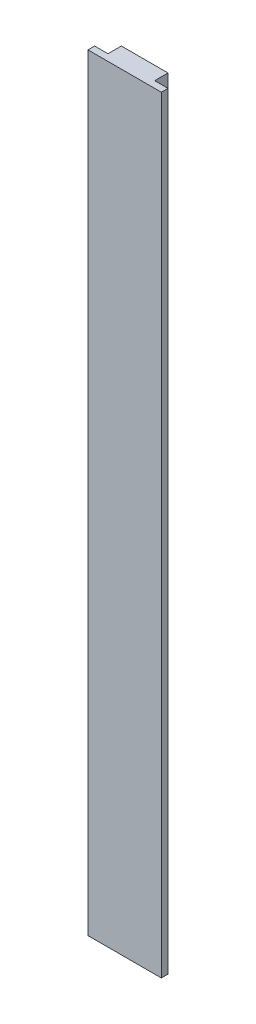
from build123d import *

# Parameters (mm, degrees)
BOSS_EXTRUDE1_DEPTH = 2300
LPATTERN1_COUNT     = 10
LPATTERN1_PITCH     = 230


with BuildPart() as part:
    # Sketch1 → Boss-Extrude1 (new body)
    with BuildSketch(Plane(origin=(0, 0, 0), x_dir=(1, 0, 0), z_dir=(0, 1, 0))):
        Polygon((-70, 10), (-70, 50), (70, 50), (70, 10), (110, 10), (110, -10), (-110, -10), (-110, 10), align=None)
    extrude(amount=BOSS_EXTRUDE1_DEPTH)

    # Sketch3 → Tap Drill for M10 Tap1 (revolve, cut)
    with BuildSketch(Plane(origin=(70, 2185, -30), x_dir=(0, 0, -1), z_dir=(0, 1, 0))):
        Polygon((0, 0), (0, 27.553657631), (4.25, 25), (4.25, 0.020977491), (4.275, 0), align=None)
    tap_drill_for_m10_tap1 = revolve(axis=Axis((76.35, 2185, -30), (-1, 0, 0)), mode=Mode.SUBTRACT)

    # LPattern1: Tap Drill for M10 Tap1 ×10
    with Locations(*[(0, -i * LPATTERN1_PITCH, 0) for i in range(1, LPATTERN1_COUNT)]):
        add(tap_drill_for_m10_tap1, mode=Mode.SUBTRACT)

    # Mirror1: Tap Drill for M10 Tap1 across plane
    add(tap_drill_for_m10_tap1.mirror(Plane(origin=(0, 0, 0), x_dir=(0, 0, 1), z_dir=(1, 0, 0))), mode=Mode.SUBTRACT)

    # Mirror1 copy 1 sketch → Mirror1 copy 1 (revolve, cut)
    with BuildSketch(Plane(origin=(-70, 1955, -30), x_dir=(0, 0, -1), z_dir=(0, 1, 0))):
        Polygon((0, 0), (0, -27.553657631), (4.25, -25), (4.25, -0.020977491), (4.275, 0), align=None)
    revolve(axis=Axis((-76.35, 1955, -30), (-1, 0, 0)), mode=Mode.SUBTRACT)

    # Mirror1 copy 2 sketch → Mirror1 copy 2 (revolve, cut)
    with BuildSketch(Plane(origin=(-70, 1725, -30), x_dir=(0, 0, -1), z_dir=(0, 1, 0))):
        Polygon((0, 0), (0, -27.553657631), (4.25, -25), (4.25, -0.020977491), (4.275, 0), align=None)
    revolve(axis=Axis((-76.35, 1725, -30), (-1, 0, 0)), mode=Mode.SUBTRACT)

    # Mirror1 copy 3 sketch → Mirror1 copy 3 (revolve, cut)
    with BuildSketch(Plane(origin=(-70, 1495, -30), x_dir=(0, 0, -1), z_dir=(0, 1, 0))):
        Polygon((0, 0), (0, -27.553657631), (4.25, -25), (4.25, -0.020977491), (4.275, 0), align=None)
    revolve(axis=Axis((-76.35, 1495, -30), (-1, 0, 0)), mode=Mode.SUBTRACT)

    # Mirror1 copy 4 sketch → Mirror1 copy 4 (revolve, cut)
    with BuildSketch(Plane(origin=(-70, 1265, -30), x_dir=(0, 0, -1), z_dir=(0, 1, 0))):
        Polygon((0, 0), (0, -27.553657631), (4.25, -25), (4.25, -0.020977491), (4.275, 0), align=None)
    revolve(axis=Axis((-76.35, 1265, -30), (-1, 0, 0)), mode=Mode.SUBTRACT)

    # Mirror1 copy 5 sketch → Mirror1 copy 5 (revolve, cut)
    with BuildSketch(Plane(origin=(-70, 1035, -30), x_dir=(0, 0, -1), z_dir=(0, 1, 0))):
        Polygon((0, 0), (0, -27.553657631), (4.25, -25), (4.25, -0.020977491), (4.275, 0), align=None)
    revolve(axis=Axis((-76.35, 1035, -30), (-1, 0, 0)), mode=Mode.SUBTRACT)

    # Mirror1 copy 6 sketch → Mirror1 copy 6 (revolve, cut)
    with BuildSketch(Plane(origin=(-70, 805, -30), x_dir=(0, 0, -1), z_dir=(0, 1, 0))):
        Polygon((0, 0), (0, -27.553657631), (4.25, -25), (4.25, -0.020977491), (4.275, 0), align=None)
    revolve(axis=Axis((-76.35, 805, -30), (-1, 0, 0)), mode=Mode.SUBTRACT)

    # Mirror1 copy 7 sketch → Mirror1 copy 7 (revolve, cut)
    with BuildSketch(Plane(origin=(-70, 575, -30), x_dir=(0, 0, -1), z_dir=(0, 1, 0))):
        Polygon((0, 0), (0, -27.553657631), (4.25, -25), (4.25, -0.020977491), (4.275, 0), align=None)
    revolve(axis=Axis((-76.35, 575, -30), (-1, 0, 0)), mode=Mode.SUBTRACT)

    # Mirror1 copy 8 sketch → Mirror1 copy 8 (revolve, cut)
    with BuildSketch(Plane(origin=(-70, 345, -30), x_dir=(0, 0, -1), z_dir=(0, 1, 0))):
        Polygon((0, 0), (0, -27.553657631), (4.25, -25), (4.25, -0.020977491), (4.275, 0), align=None)
    revolve(axis=Axis((-76.35, 345, -30), (-1, 0, 0)), mode=Mode.SUBTRACT)

    # Mirror1 copy 9 sketch → Mirror1 copy 9 (revolve, cut)
    with BuildSketch(Plane(origin=(-70, 115, -30), x_dir=(0, 0, -1), z_dir=(0, 1, 0))):
        Polygon((0, 0), (0, -27.553657631), (4.25, -25), (4.25, -0.020977491), (4.275, 0), align=None)
    revolve(axis=Axis((-76.35, 115, -30), (-1, 0, 0)), mode=Mode.SUBTRACT)


solid = part.part
